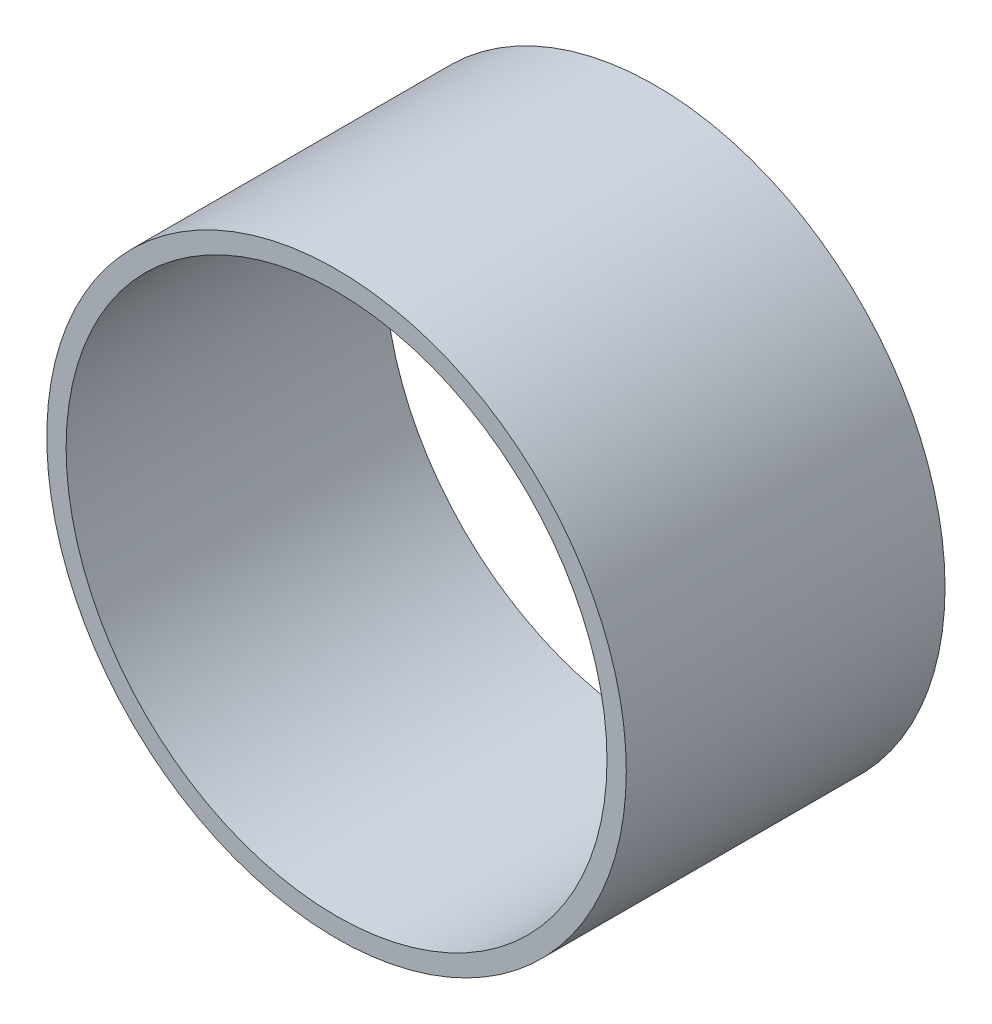
from build123d import *

# Parameters (mm, degrees)
SKETCH1_R           = 30
SKETCH1_R_2         = 28
BOSS_EXTRUDE1_DEPTH = 33


with BuildPart() as part:
    # Sketch1 → Boss-Extrude1 (new body)
    with BuildSketch(Plane.XY):
        Circle(SKETCH1_R)
        Circle(SKETCH1_R_2, mode=Mode.SUBTRACT)
    extrude(amount=BOSS_EXTRUDE1_DEPTH)


solid = part.part
